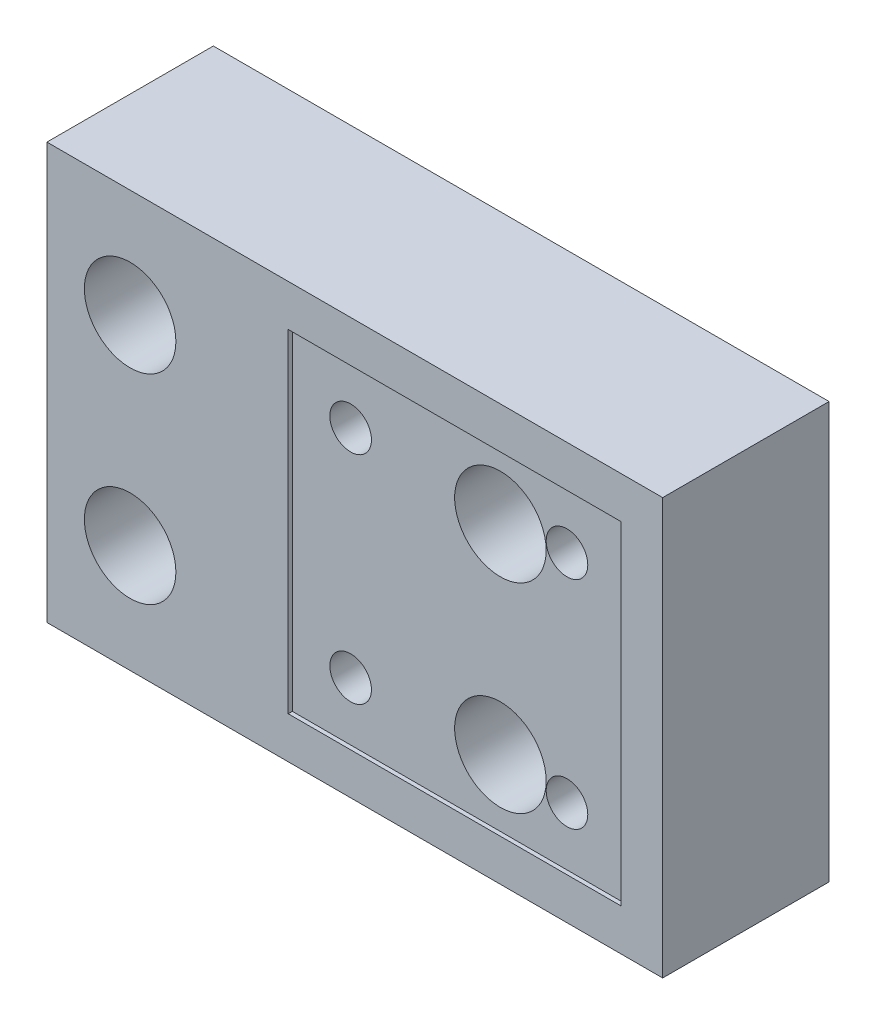
from build123d import *

# Parameters (mm, degrees)
SKETCH1_W           = 74
SKETCH1_H           = 50
BOSS_EXTRUDE1_DEPTH = 20
SKETCH2_W           = 40
SKETCH2_H           = 40
CUT_EXTRUDE1_DEPTH  = 0.5
SKETCH3_W           = 10
SKETCH3_H           = 40
BOSS_EXTRUDE2_DEPTH = 3
CHAMFER1_SIZE       = 2
SKETCH4_R           = 3.3
SKETCH4_R_2         = 2.5
CUT_EXTRUDE2_DEPTH  = 51.229473419
SKETCH5_R           = 5.5
CUT_EXTRUDE3_DEPTH  = 15


with BuildPart() as part:
    # Sketch1 → Boss-Extrude1 (new body)
    with BuildSketch(Plane.XY):
        Rectangle(SKETCH1_W, SKETCH1_H)
    extrude(amount=BOSS_EXTRUDE1_DEPTH)

    # Sketch2 → Cut-Extrude1 (cut)
    with BuildSketch(Plane.XY.offset(20)):
        with Locations((12, 0)):
            Rectangle(SKETCH2_W, SKETCH2_H)
    extrude(amount=-CUT_EXTRUDE1_DEPTH, mode=Mode.SUBTRACT)

    # Sketch3 → Boss-Extrude2 (add)
    with BuildSketch(Plane(origin=(0, 0, 0), x_dir=(-1, 0, 0), z_dir=(0, 0, -1))):
        with Locations((-17, 0)):
            Rectangle(SKETCH3_W, SKETCH3_H)
        with Locations((27, 0)):
            Rectangle(SKETCH3_W, SKETCH3_H)
    extrude(amount=BOSS_EXTRUDE2_DEPTH)

    # Chamfer1
    chamfer1_edges = [part.edges().sort_by_distance(p)[0] for p in [
        (22, 20, -1.5),
        (22, -20, -1.5),
        (12, -20, -1.5),
        (12, 20, -1.5),
        (-22, 20, -1.5),
        (-22, -20, -1.5),
        (-32, -20, -1.5),
        (-32, 20, -1.5),
    ]]
    chamfer(chamfer1_edges, length=CHAMFER1_SIZE)

    # Sketch4 → Cut-Extrude2 (cut, through all)
    with BuildSketch(Plane(origin=(0, 0, -3), x_dir=(-1, 0, 0), z_dir=(0, 0, -1))):
        with Locations((-17, 12)):
            Circle(SKETCH4_R)
        with Locations((27, 12)):
            Circle(SKETCH4_R)
        with Locations((-25, 13)):
            Circle(SKETCH4_R_2)
        with Locations((1, 13)):
            Circle(SKETCH4_R_2)
        with Locations((1, -13)):
            Circle(SKETCH4_R_2)
        with Locations((-25, -13)):
            Circle(SKETCH4_R_2)
        with Locations(Location((27, -12, 0), (0, 0, 180))):
            Circle(SKETCH4_R)
        with Locations(Location((-17, -12, 0), (0, 0, 180))):
            Circle(SKETCH4_R)
    extrude(amount=-CUT_EXTRUDE2_DEPTH, mode=Mode.SUBTRACT)

    # Sketch5 → Cut-Extrude3 (cut)
    with BuildSketch(Plane.XY.offset(20)):
        with Locations((-27, 12)):
            Circle(SKETCH5_R)
        with Locations((-27, -12)):
            Circle(SKETCH5_R)
        with Locations((17, 12)):
            Circle(SKETCH5_R)
        with Locations((17, -12)):
            Circle(SKETCH5_R)
    extrude(amount=-CUT_EXTRUDE3_DEPTH, mode=Mode.SUBTRACT)


solid = part.part
